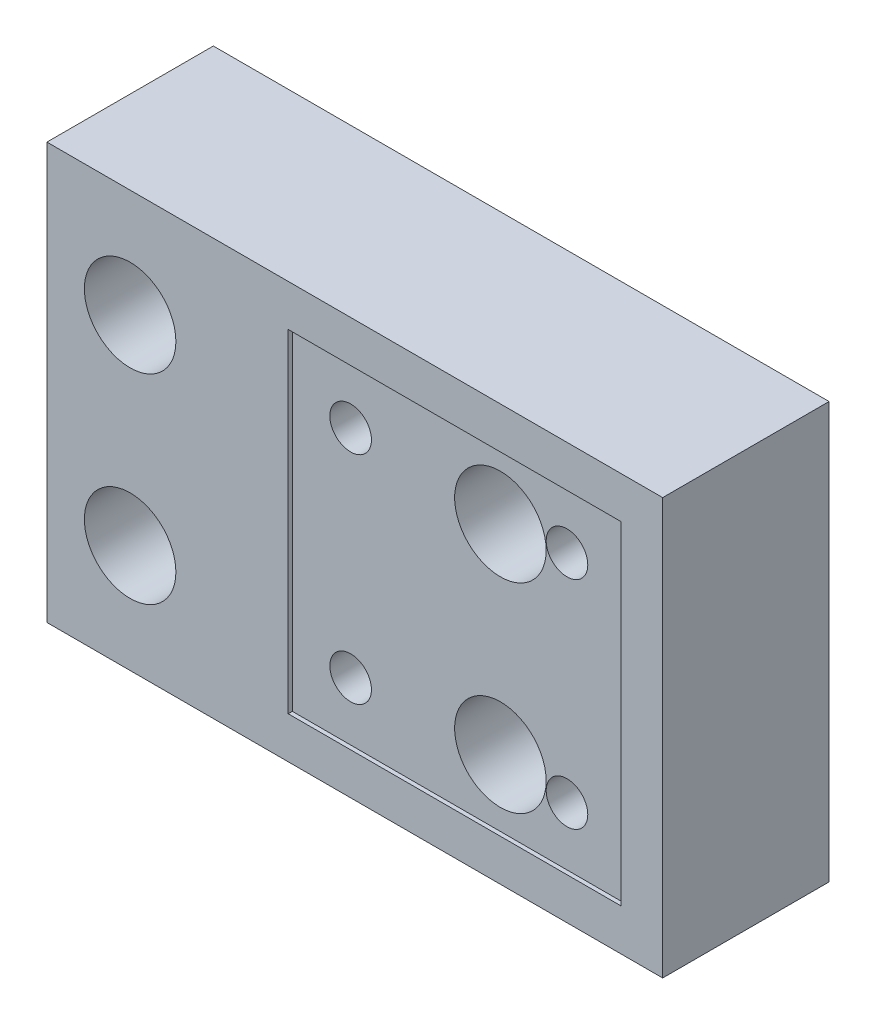
SolidWorks part; units mm, degrees
ref_plane "Front Plane" through (0, 0, 0) normal (0, 0, 1) x (1, 0, 0)
ref_plane "Top Plane" through (0, 0, 0) normal (0, 1, 0) x (1, 0, 0)
ref_plane "Right Plane" through (0, 0, 0) normal (1, 0, 0) x (0, 0, -1)
sketch "Sketch1" plane through (0, 0, 0) normal (0, 0, 1) x (1, 0, 0)
  line L1 (37, 25) -> (-37, 25)
  line L2 (37, 25) -> (37, -25)
  line L3 (37, -25) -> (-37, -25)
  line L4 (-37, 25) -> (-37, -25)
  line L5 (37, 25) -> (-37, -25) construction
  line L6 (37, -25) -> (-37, 25) construction
  point P0 (0, 0)
  dimension "D1" = 74
  dimension "D2" = 50
extrude "Boss-Extrude1" add sketch "Sketch1" along normal blind 20
sketch "Sketch2" plane through (0, 0, 20) normal (0, 0, 1) x (1, 0, 0)
  line L0 (37, -25) -> (37, 25) construction
  line L1 (32, -20) -> (-8, -20)
  line L2 (32, -20) -> (32, 20)
  line L3 (32, 20) -> (-8, 20)
  line L4 (-8, -20) -> (-8, 20)
  line L5 (32, -20) -> (-8, 20) construction
  line L6 (32, 20) -> (-8, -20) construction
  point P0 (12, 0)
  dimension "D1" = 40
  dimension "D2" = 40
  dimension "D3" = 5
extrude "Cut-Extrude1" cut sketch "Sketch2" against normal blind 0.5
sketch "Sketch3" plane through (0, 0, 0) normal (0, 0, -1) x (-1, 0, 0)
  line L0 (-37, -25) -> (-37, 25) construction
  line L1 (-12, -20) -> (-22, -20)
  line L2 (-12, -20) -> (-12, 20)
  line L3 (-12, 20) -> (-22, 20)
  line L4 (-22, -20) -> (-22, 20)
  line L5 (-12, -20) -> (-22, 20) construction
  line L6 (-12, 20) -> (-22, -20) construction
  line L7 (32, -20) -> (22, -20)
  line L8 (32, -20) -> (32, 20)
  line L9 (32, 20) -> (22, 20)
  line L10 (22, -20) -> (22, 20)
  line L11 (32, -20) -> (22, 20) construction
  line L12 (32, 20) -> (22, -20) construction
  line L13 (37, 25) -> (37, -25) construction
  point P0 (-17, 0)
  point P5 (27, 0)
  dimension "D1" = 10
  dimension "D2" = 40
  dimension "D3" = 10
  dimension "D4" = 40
  dimension "D5" = 15
  dimension "D6" = 5
extrude "Boss-Extrude2" add sketch "Sketch3" along normal blind 3
chamfer "Chamfer1" distance 2 angle 45 8 edges at (-32, 20, -1.5) (-22, 20, -1.5) (12, 20, -1.5) (22, 20, -1.5) (-22, -20, -1.5) (-32, -20, -1.5) (12, -20, -1.5) (22, -20, -1.5)
sketch "Sketch4" plane through (0, 0, -3) normal (0, 0, -1) x (-1, 0, 0)
  line L0 (-37, -25) -> (-37, 25) construction
  line L1 (-37, 25) -> (37, 25) construction
  line L2 (0, 0) -> (13.6825, 0) construction
  circle A0 centre (-17, 12) radius 3.3
  circle A1 centre (27, 12) radius 3.3
  circle A2 centre (-25, 13) radius 2.5
  circle A3 centre (1, 13) radius 2.5
  circle A4 centre (1, -13) radius 2.5
  circle A5 centre (-25, -13) radius 2.5
  circle A6 centre (27, -12) radius 3.3
  circle A7 centre (-17, -12) radius 3.3
  dimension "D4" = 5
  dimension "D5" = 6.6
  dimension "D1" = 44
  dimension "D2" = 26
  dimension "D3" = 12
  dimension "D6" = 13
  dimension "D7" = 12
  dimension "D8" = 20
extrude "Cut-Extrude2" cut sketch "Sketch4" against normal through all
sketch "Sketch5" plane through (0, 0, 20) normal (0, 0, 1) x (1, 0, 0)
  circle A0 centre (-27, 12) radius 5.5
  circle A1 centre (-27, -12) radius 5.5
  circle A2 centre (17, 12) radius 5.5
  circle A3 centre (17, -12) radius 5.5
  dimension "D1" = 11
extrude "Cut-Extrude3" cut sketch "Sketch5" against normal blind 15
